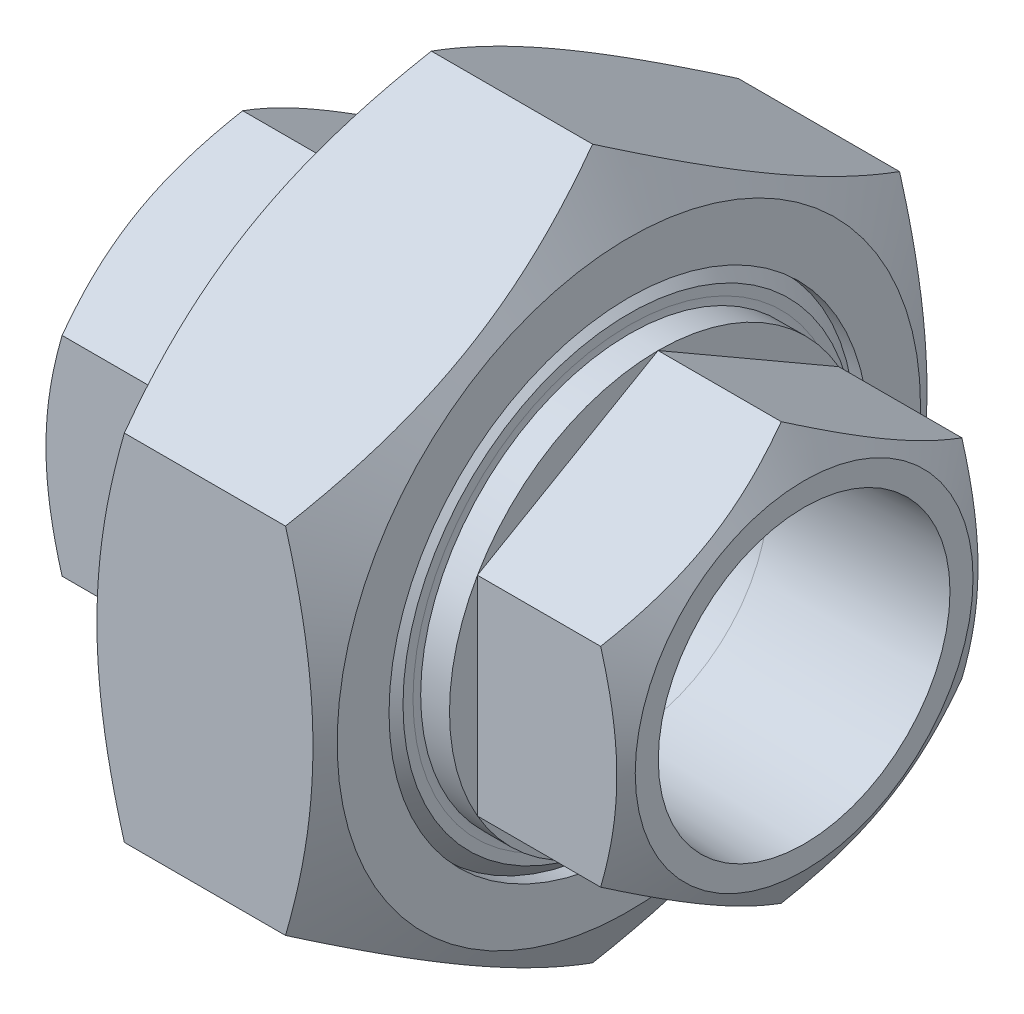
SolidWorks part; units mm, degrees
material "KTH350-10"
ref_plane "前视基准面" through (0, 0, 0) normal (0, 0, 1) x (1, 0, 0)
ref_plane "上视基准面" through (0, 0, 0) normal (0, 1, 0) x (1, 0, 0)
ref_plane "右视基准面" through (0, 0, 0) normal (1, 0, 0) x (0, 0, -1)
sketch "草图1" plane through (0, 0, 0) normal (0, 0, 1) x (1, 0, 0)
  line L0 (0, 0) -> (0, 23.805) construction
  line L1 (0, 0) -> (29, 0) construction
  line L2 (29, 20.7) -> (11.6, 20.7)
  line L3 (11.6, 20.7) -> (11.6, 23.805)
  line L4 (11.6, 23.805) -> (0, 23.805)
  line L5 (0, 23.805) -> (0, 27.324)
  line L6 (0, 27.324) -> (-11.6, 27.324)
  line L7 (-11.6, 27.324) -> (-11.6, 20.7)
  line L8 (-11.6, 20.7) -> (-29, 20.7)
  line L9 (-29, 20.7) -> (-29, 14.4776)
  line L10 (-29, 14.4776) -> (-11.6, 13.87)
  line L11 (-11.6, 13.87) -> (11.6, 13.87)
  line L12 (11.6, 13.87) -> (29, 14.4776)
  line L13 (29, 14.4776) -> (29, 20.7)
  line L14 (-11.6, 27.324) -> (-11.6, 35.19) construction
  line L15 (-11.6, 35.19) -> (11.6, 35.19) construction
  line L16 (11.6, 35.19) -> (11.6, 23.805) construction
revolve "旋转1" add sketch "草图1" angle 360 about L1
chamfer "倒角1" distance 1.387 angle 45 2 edges at (-11.6, 0, 27.324) (11.6, 0, 23.805)
sketch "草图3" plane through (0, 0, 0) normal (0, 0, 1) x (1, 0, 0)
  line L0 (-11.6, 27.324) -> (-11.6, 35.19)
  line L1 (-11.6, 35.19) -> (11.6, 35.19)
  line L2 (11.6, 35.19) -> (11.6, 23.805)
  line L3 (11.6, 23.805) -> (0, 23.805)
  line L4 (0, 23.805) -> (0, 27.324)
  line L5 (0, 27.324) -> (-11.6, 27.324)
  line L6 (0, 0) -> (14.2687, 0) construction
  line L7 (0, 0) -> (29, 0) construction
revolve "旋转2" add sketch "草图3" angle 360 about L6
sketch "草图4" plane through (29, 0, 0) normal (1, 0, 0) x (0, 0, -1)
  line L1 (0, 20.7) -> (-17.9267, 10.35)
  line L2 (-17.9267, 10.35) -> (-17.9267, -10.35)
  line L3 (-17.9267, -10.35) -> (0, -20.7)
  line L4 (0, -20.7) -> (17.9267, -10.35)
  line L5 (17.9267, -10.35) -> (17.9267, 10.35)
  line L6 (17.9267, 10.35) -> (0, 20.7)
  circle A0 centre (0, 0) radius 17.9267 construction
  circle A2 centre (0, 0) radius 20.7 construction
  circle A3 centre (0, 0) radius 23.805 construction
  circle A4 centre (0, 0) radius 23.805
  dimension "D1" = 35.8535
extrude "切除-拉伸1" cut sketch "草图4" against normal blind 14.5
sketch "草图5" plane through (29, 0, 0) normal (1, 0, 0) x (0, 0, -1)
  circle A0 centre (0, 0) radius 16.767
extrude "切除-拉伸2" cut sketch "草图5" against normal blind 11.6 draft 60 flip side to cut
sketch "草图6" plane through (0, 0, 0) normal (0, 0, 1) x (1, 0, 0)
  line L0 (11.6, 20.7) -> (11.6, 23.805) construction
  line L1 (11.6, -35.19) -> (11.6, 35.19) construction
  line L2 (18.8996, 14.1249) -> (11.6, 14.1249)
  line L3 (11.6, 14.1249) -> (11.6, 21.4245)
  line L4 (0, 0) -> (29, 0) construction
  line L5 (29, 14.4776) -> (11.6, 13.87) construction
  arc A0 (11.6, 21.4245) -> (18.8996, 14.1249) centre (18.8996, 21.4245) ccw
revolve "旋转3" add sketch "草图6" angle 360 about L4
sketch "草图8" plane through (11.6, 0, 0) normal (1, 0, 0) x (0, 0, -1)
  line L1 (0, 35.19) -> (-30.4754, 17.595)
  line L2 (-30.4754, 17.595) -> (-30.4754, -17.595)
  line L3 (-30.4754, -17.595) -> (0, -35.19)
  line L4 (0, -35.19) -> (30.4754, -17.595)
  line L5 (30.4754, -17.595) -> (30.4754, 17.595)
  line L6 (30.4754, 17.595) -> (0, 35.19)
  circle A0 centre (0, 0) radius 30.4754 construction
  circle A1 centre (0, 0) radius 35.19 construction
  circle A2 centre (0, 0) radius 38.709
extrude "切除-拉伸3" cut sketch "草图8" against normal through all
sketch "草图10" plane through (11.6, 0, 0) normal (1, 0, 0) x (0, 0, -1)
  circle A0 centre (0, 0) radius 28.9517
extrude "切除-拉伸4" cut sketch "草图10" against normal blind 10 draft 60 flip side to cut
mirror "镜向7" about plane through (0, 0, 0) normal (1, 0, 0) of "切除-拉伸4", "切除-拉伸2", "切除-拉伸1", "旋转3"
equation "\"D3@草图1\" = \"L@草图1\" * 0.4"
equation "\"D4@草图1\" = \"D@草图1\"*1.15"
equation "\"D5@草图1\" = \"D@草图1\"*1.32"
equation "\"D6@草图1\" = \"D@草图1\"*1.7"
equation "\"D1@倒角1\" = \"d2@草图1\"*0.05"
equation "\"D1@草图5\" = \"D@草图1\"*0.81"
equation "\"D1@切除-拉伸1\" = \"L@草图1\"*0.25"
equation "\"D1@草图6\" = \"D4@草图1\"*0.9"
equation "\"D1@切除-拉伸2\" = \"L@草图1\"*0.2"
equation "\"D1@草图8\" = \"D6@草图1\"*1.1"
equation "\"D1@草图10\" = \"D2@草图8\"*0.95"
